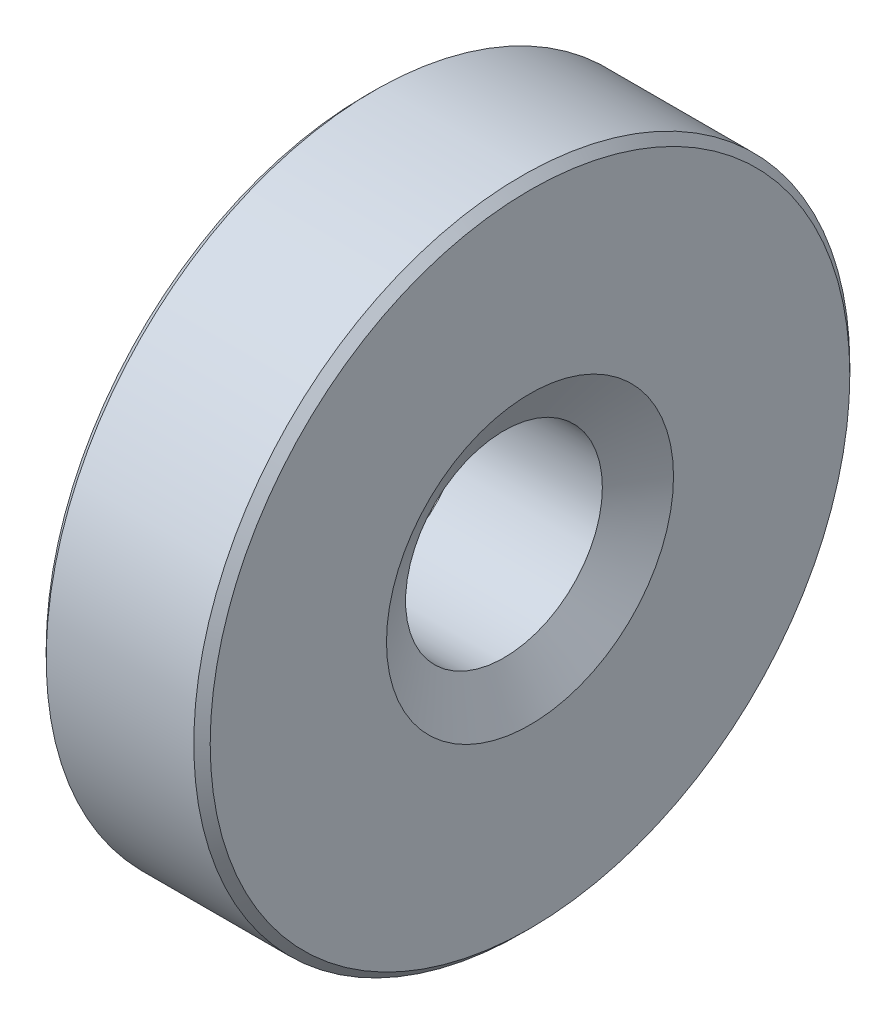
from build123d import *

# Parameters (mm, degrees)
SKETCH1_R          = 40
EXTRUDE1_DEPTH     = 20
SKETCH2_R          = 12
CUT_EXTRUDE1_DEPTH = 61
CHAMFER1_SIZE      = 1
CHAMFER2_SIZE      = 5.5
CHAMFER2_SIZE2     = 3.175426481


with BuildPart() as part:
    # Sketch1 → Extrude1 (new body)
    with BuildSketch(Plane(origin=(0, 0, 0), x_dir=(0, 0, -1), z_dir=(1, 0, 0))):
        Circle(SKETCH1_R)
    extrude(amount=EXTRUDE1_DEPTH)

    # Sketch2 → Cut-Extrude1 (cut, through all)
    with BuildSketch(Plane(origin=(20, 0, 0), x_dir=(0, 0, -1), z_dir=(1, 0, 0))):
        Circle(SKETCH2_R)
    extrude(amount=-CUT_EXTRUDE1_DEPTH, mode=Mode.SUBTRACT)

    # Chamfer1
    chamfer1_edges = [part.edges().sort_by_distance(p)[0] for p in [
        (0, 0, 40),
        (20, 0, 40),
    ]]
    chamfer(chamfer1_edges, length=CHAMFER1_SIZE)

    # Chamfer2
    chamfer2_edges = [part.edges().sort_by_distance(p)[0] for p in [
        (20, 0, 12),
    ]]
    chamfer2_side = [part.faces().sort_by_distance(p)[0] for p in [
        (20, 0, 37.896913421),
    ]]
    chamfer(chamfer2_edges, length=CHAMFER2_SIZE, length2=CHAMFER2_SIZE2, reference=chamfer2_side[0])


solid = part.part
